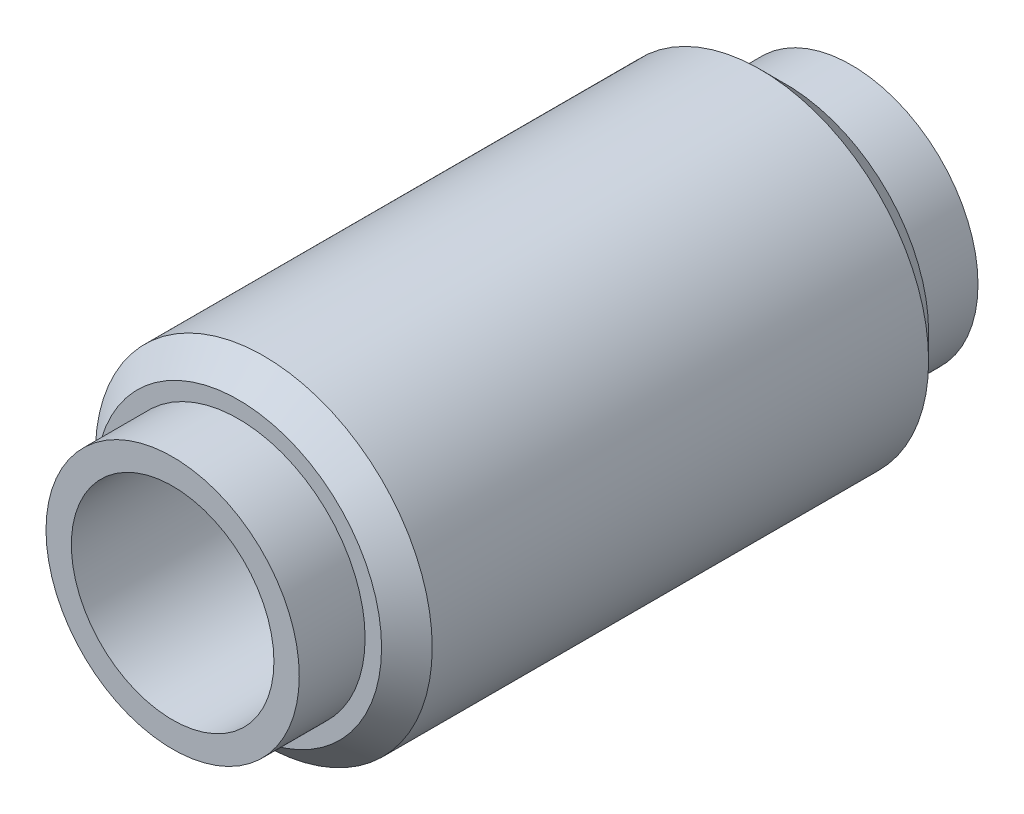
from build123d import *

# Parameters (mm, degrees)
SKETCH1_R           = 50
BOSS_EXTRUDE1_DEPTH = 26
SKETCH2_R           = 66.5
BOSS_EXTRUDE2_DEPTH = 216
SKETCH3_R           = 50
BOSS_EXTRUDE3_DEPTH = 26
SKETCH4_R           = 40
CUT_EXTRUDE1_DEPTH  = 79
CUT_EXTRUDE2_START  = -79
SKETCH5_R           = 40
CUT_EXTRUDE2_DEPTH  = 79
SKETCH6_R           = 36.5
CUT_EXTRUDE3_DEPTH  = 212.1054239
CHAMFER1_SIZE       = 10
CHAMFER2_SIZE       = 10


with BuildPart() as part:
    # Sketch1 → Boss-Extrude1 (new body)
    with BuildSketch(Plane.XY):
        with Locations(Location((0, 0, 0), (0, 0, 180))):
            Circle(SKETCH1_R)
    extrude(amount=BOSS_EXTRUDE1_DEPTH)

    # Sketch2 → Boss-Extrude2 (add)
    with BuildSketch(Plane.XY.offset(26)):
        Circle(SKETCH2_R)
    extrude(amount=BOSS_EXTRUDE2_DEPTH)

    # Sketch3 → Boss-Extrude3 (add)
    with BuildSketch(Plane.XY.offset(242)):
        with Locations(Location((0, 0, 0), (0, 0, 180))):
            Circle(SKETCH3_R)
    extrude(amount=BOSS_EXTRUDE3_DEPTH)

    # Sketch4 → Cut-Extrude1 (cut)
    with BuildSketch(Plane.XY.offset(268)):
        Circle(SKETCH4_R)
    extrude(amount=-CUT_EXTRUDE1_DEPTH, mode=Mode.SUBTRACT)

    # Sketch5 → Cut-Extrude2 (cut)
    with BuildSketch(Plane(origin=(0, 0, 0), x_dir=(-1, 0, 0), z_dir=(0, 0, -1)).offset(CUT_EXTRUDE2_START)):
        with Locations(Location((0, 0, 0), (0, 0, 180))):
            Circle(SKETCH5_R)
    extrude(amount=CUT_EXTRUDE2_DEPTH, mode=Mode.SUBTRACT)

    # Sketch6 → Cut-Extrude3 (cut, through all)
    with BuildSketch(Plane(origin=(0, 0, 79), x_dir=(-1, 0, 0), z_dir=(0, 0, -1))):
        Circle(SKETCH6_R)
    extrude(amount=-CUT_EXTRUDE3_DEPTH, mode=Mode.SUBTRACT)

    # Chamfer1
    chamfer1_edges = [part.edges().sort_by_distance(p)[0] for p in [
        (-66.5, 0, 242),
    ]]
    chamfer(chamfer1_edges, length=CHAMFER1_SIZE)

    # Chamfer2
    chamfer2_edges = [part.edges().sort_by_distance(p)[0] for p in [
        (-66.5, 0, 26),
    ]]
    chamfer(chamfer2_edges, length=CHAMFER2_SIZE)


solid = part.part
